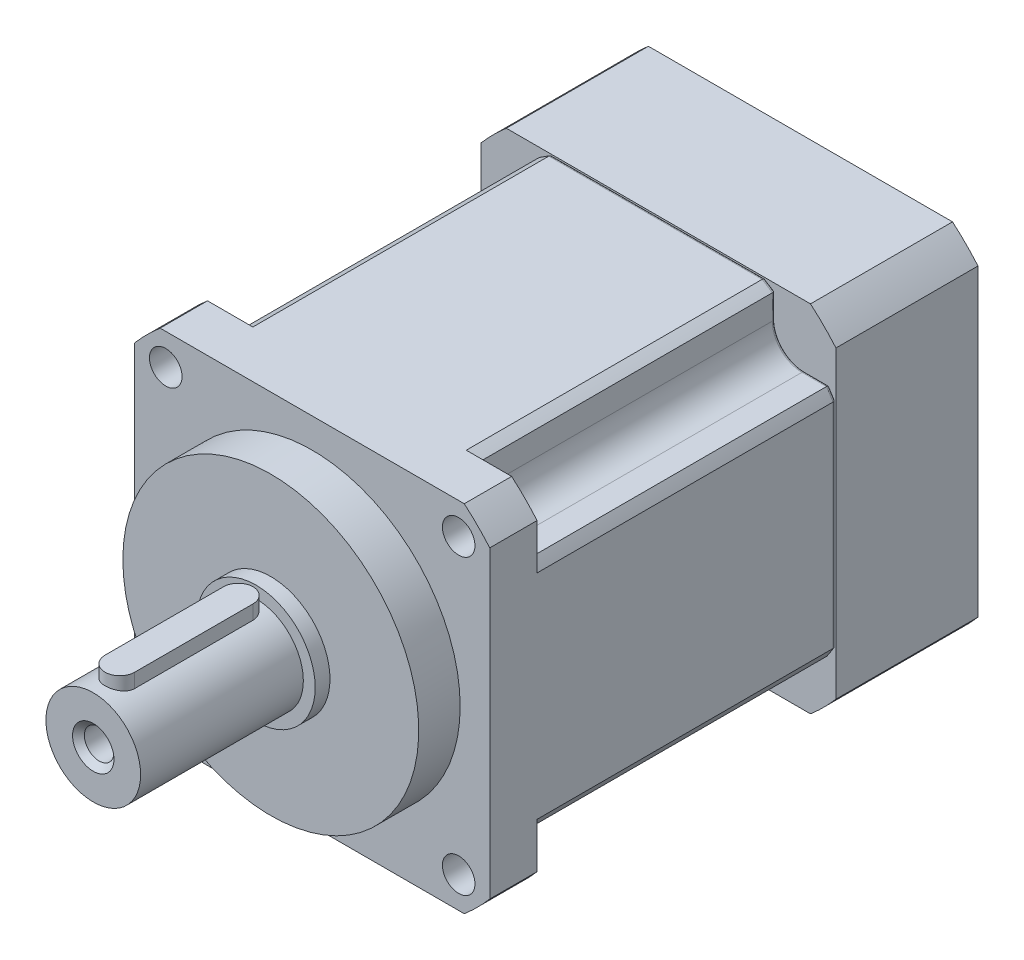
SolidWorks part; units mm, degrees
ref_plane "前视基准面" through (0, 0, 0) normal (0, 0, 1) x (1, 0, 0)
ref_plane "上视基准面" through (0, 0, 0) normal (0, 1, 0) x (1, 0, 0)
ref_plane "右视基准面" through (0, 0, 0) normal (1, 0, 0) x (0, 0, -1)
sketch "草图1" plane through (0, 0, 0) normal (0, 0, 1) x (1, 0, 0)
  circle A0 centre (0, 0) radius 25
  dimension "D5" = 50
extrude "第一段" add sketch "草图1" along normal blind 37
ref_plane "基准面1" through (0, 0, 7) normal (0, 0, -1) x (-1, 0, 0)
sketch "草图2" plane through (0, 0, 7) normal (0, 0, -1) x (-1, 0, 0)
  circle A0 centre (0, 0) radius 10
  dimension "D4" = 20
extrude "切除-拉伸1" cut sketch "草图2" against normal through all flip side to cut
sketch "草图3" plane through (0, 0, 37) normal (0, 0, 1) x (1, 0, 0)
  circle A0 centre (0, 0) radius 8
extrude "切除-拉伸2" cut sketch "草图3" against normal blind 27.5 flip side to cut
ref_plane "基准面2" through (0, -8, 0) normal (0, 1, 0) x (-1, 0, 0)
ref_plane "基准面6" through (0, 10, 0) normal (0, 1, 0) x (-1, 0, 0)
sketch "草图4" plane through (0, 10, 0) normal (0, 1, 0) x (-1, 0, 0)
  line L0 (0, 37) -> (0, 35) construction
  line L1 (8, 37) -> (-8, 37) construction
  line L2 (0, 35) -> (0, 10) construction
  line L5 (-2.5, 32.5) -> (-2.5, 12.5)
  line L6 (2.5, 12.5) -> (2.5, 32.5)
  arc A0 (2.5, 32.5) -> (-2.5, 32.5) centre (0, 32.5) ccw
  arc A1 (-2.5, 12.5) -> (2.5, 12.5) centre (0, 12.5) ccw
  dimension "B1" = 5
  dimension "L2" = 2
  dimension "L1" = 25
extrude "凸台-拉伸2" add sketch "草图4" against normal up to next
sketch "草图6" plane through (0, 0, 0) normal (0, 0, -1) x (-1, 0, 0)
  line L1 (-30, -30) -> (30, -30)
  line L2 (-30, -30) -> (-30, 30)
  line L3 (-30, 30) -> (30, 30)
  line L4 (30, -30) -> (30, 30)
  line L5 (-30, -30) -> (30, 30) construction
  line L6 (-30, 30) -> (30, -30) construction
  point P0 (0, 0)
extrude "第二段" add sketch "草图6" along normal blind 58.5
ref_plane "基准面3" through (0, 0, -8) normal (0, 0, 1) x (1, 0, 0)
sketch "草图7" plane through (0, 0, -8) normal (0, 0, 1) x (1, 0, 0)
  line L0 (0, 0) -> (35, 0) construction
  line L1 (0, 0) -> (24.7487, 24.7487) construction
  line L2 (24.7487, 19.7487) -> (28.8961, 19.7487)
  line L3 (19.7487, 24.7487) -> (19.7487, 28.8961)
  line L5 (30, 30) -> (30, -30) construction
  line L7 (30, 30) -> (30, 18.0278)
  line L8 (18.0278, 30) -> (30, 30)
  circle A0 centre (0, 0) radius 35 construction
  arc A1 (19.7487, 24.7487) -> (24.7487, 19.7487) centre (24.7487, 24.7487) ccw
  arc A3 (30, 18.0278) -> (28.8961, 19.7487) centre (0, 0) ccw
  arc A4 (19.7487, 28.8961) -> (18.0278, 30) centre (0, 0) ccw
  dimension "D61" = 70
  dimension "D62" = 5
  dimension "D63" = 70
  dimension "D4" = 45
extrude "切除-拉伸8" cut sketch "草图7" against normal through all
pattern_circular "阵列(圆周)2" count 4 over 360 about axis through (0, 0, 0) along (0, 0, 1) of "切除-拉伸8"
sketch "草图9" plane through (0, 0, 0) normal (0, 0, 1) x (1, 0, 0)
  line L0 (0, 0) -> (35, 0) construction
  line L1 (0, 0) -> (24.7487, 24.7487) construction
  circle A0 centre (0, 0) radius 35 construction
  circle A1 centre (24.7487, 24.7487) radius 2.75
  dimension "D1" = 70
  dimension "D3" = 45
  dimension "D2" = 5.5
extrude "切除-拉伸6" cut sketch "草图9" against normal up to next
pattern_circular "阵列(圆周)1" count 4 over 360 about axis through (0, 0, 0) along (0, 0, 1) of "切除-拉伸6"
sketch "草图10" plane through (0, 0, 0) normal (0, 0, 1) x (1, 0, 0)
  circle A0 centre (0, 0) radius 39.5
extrude "切除-拉伸7" cut sketch "草图10" against normal through all flip side to cut
fillet "圆角3" radius 0.5 24 edges at (0, 30, -58.5) (-30, 0, -58.5) (0, -30, -58.5) (30, 0, -58.5) (-29.4606, -18.8963, -58.5) (-26.8224, -19.7487, -58.5) (-21.2132, -21.2132, -58.5) (-19.7487, -26.8224, -58.5) (-18.8963, -29.4606, -58.5) (18.8963, -29.4606, -58.5) (19.7487, -26.8224, -58.5) (21.2132, -21.2132, -58.5) (26.8224, -19.7487, -58.5) (29.4606, -18.8963, -58.5) (29.4606, 18.8963, -58.5) (26.8224, 19.7487, -58.5) (21.2132, 21.2132, -58.5) (19.7487, 26.8224, -58.5) (18.8963, 29.4606, -58.5) (-18.8963, 29.4606, -58.5) (-19.7487, 26.8224, -58.5) (-21.2132, 21.2132, -58.5) (-26.8224, 19.7487, -58.5) (-29.4606, 18.8963, -58.5)
sketch "草图15" plane through (0, 0, -58.5) normal (0, 0, -1) x (-1, 0, 0)
  line L1 (-30, 30) -> (30, 30)
  line L2 (-30, 30) -> (-30, -30)
  line L3 (-30, -30) -> (30, -30)
  line L4 (30, 30) -> (30, -30)
  line L5 (-30, 30) -> (30, -30) construction
  line L6 (-30, -30) -> (30, 30) construction
  point P0 (0, 0)
extrude "第三段" add sketch "草图15" along normal blind 24
sketch "草图21" plane through (0, 0, -82.5) normal (0, 0, -1) x (-1, 0, 0)
  circle A0 centre (0, 0) radius 39.5
extrude "切除-拉伸10" cut sketch "草图21" against normal blind 24 flip side to cut
sketch "草图22" plane through (0, 0, -82.5) normal (0, 0, -1) x (-1, 0, 0)
  circle A0 centre (0, 0) radius 25
  dimension "D51" = 50
extrude "切除-拉伸11" cut sketch "草图22" against normal blind 5
sketch "草图30" plane through (0, 0, -82.5) normal (0, 0, -1) x (-1, 0, 0)
  circle A0 centre (0, 0) radius 7
  dimension "D31" = 14
extrude "切除-拉伸15" cut sketch "草图30" against normal blind 32
hole_wizard "M5 螺纹孔1" positions "草图32" profile "草图31" tap size "M5" standard "GB"
sketch "草图32" plane through (0, 0, 37) normal (0, 0, 1) x (1, 0, 0)
  point P1 (0, 0)
sketch "草图31" plane through (0, 0, 37) normal (1, 0, 0) x (0, -1, 0)
  line L0 (0, 0) -> (0, 15.2017)
  line L1 (0, 15.2017) -> (2, 14)
  line L2 (2, 14) -> (2, 12)
  line L3 (2, 12) -> (2.5, 12)
  line L5 (2.5, 12) -> (2.5, 1)
  line L6 (2.5, 1) -> (3.5, 0)
  line L7 (3.5, 0) -> (0, 0)
  line L8 (-2.5, 1) -> (-3.5, 0) construction
  line L10 (0, 15.2017) -> (-2, 14) construction
  line L11 (0, -6.35) -> (0, 107.95) construction
hole_wizard "M5 螺纹孔2" positions "草图35" profile "草图34" tap size "M5" standard "GB"
sketch "草图35" plane through (0, 0, -82.5) normal (0, 0, -1) x (-1, 0, 0)
  line L0 (0, 0) -> (35, 0) construction
  line L3 (0, 0) -> (24.7487, 24.7487) construction
  circle A0 centre (0, 0) radius 35 construction
  point P1 (24.7487, 24.7487)
  dimension "D11" = 70
  dimension "D2" = 45
sketch "草图34" plane through (-24.7487, 24.7487, -82.5) normal (1, 0, 0) x (0, 1, 0)
  line L0 (0, 0) -> (0, 13.2017)
  line L1 (0, 13.2017) -> (2, 12)
  line L2 (2, 12) -> (2, 10)
  line L3 (2, 10) -> (2.5, 10)
  line L4 (2.5, 10) -> (2.5, 0)
  line L5 (2.5, 0) -> (0, 0)
  line L10 (0, 13.2017) -> (-2, 12) construction
  line L11 (0, -6.35) -> (0, 107.95) construction
pattern_circular "阵列(圆周)3" count 4 over 360 about axis through (0, 0, 0) along (0, 0, 1) of "M5 螺纹孔2"
equation "\"D1@草图6\" = \"A1@草图6\""
equation "\"D1@切除-拉伸10\" = \"L61@第三段\""
equation "\"D1@草图15\" = \"A2@草图15\""
equation "\"D1@基准面2\" = \"D3@草图3\" / 2"
equation "\"输出法兰圆角切除@草图10\" = \"A1@草图6\" * 1.4 - 5"
equation "\"输入法兰圆角切除@草图21\" = \"A2@草图15\" * 1.4 - 5"
equation "\"近端锥形沉头孔直径@草图31\" = \"C1@草图31\" + 2"
equation "\"螺纹孔钻头深度@草图31\" = \"螺纹深度@草图31\" + 2"
equation "\"螺纹孔钻头直径@草图31\" = \"C1@草图31\" - 1"
equation "\"螺纹孔钻头直径@草图34\" = \"D21@草图34\" - 1"
equation "\"螺纹孔钻头深度@草图34\" = \"螺纹深度@草图34\" + 2"
